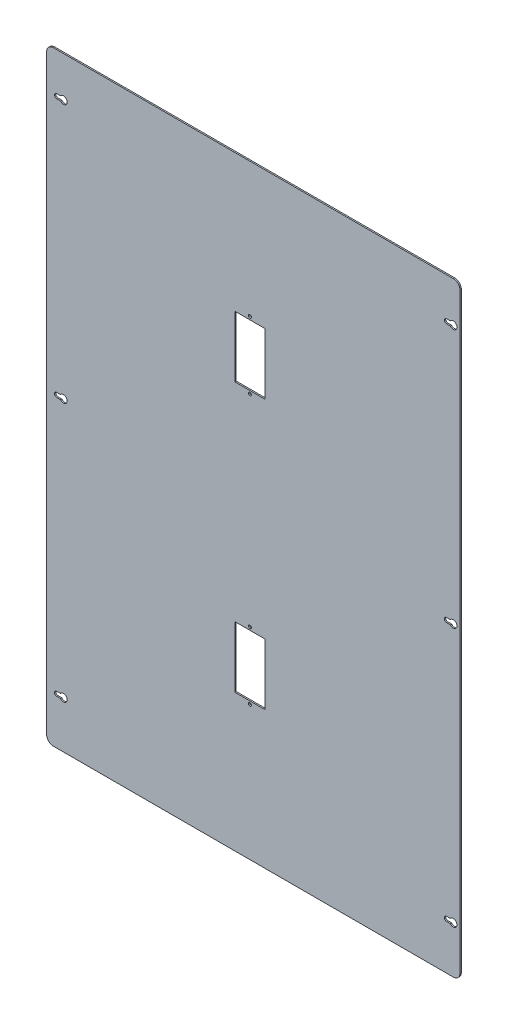
from build123d import *

# Parameters (mm, degrees)
SKETCH1_W            = 615
SKETCH1_H            = 900
BOSS_EXTRUDE1_DEPTH  = 2
SKETCH7_W            = 45
SKETCH7_H            = 91
CUT_EXTRUDE4_DEPTH   = 546.03233849
SKETCH8_R            = 2.25
CUT_EXTRUDE5_DEPTH   = 546.03233849
FILLET3_R            = 10
CUT_EXTRUDE6_DEPTH   = 10
LPATTERN1_COUNT      = 3
LPATTERN1_PITCH      = 385
LPATTERN1_COUNT_DIR2 = 2
LPATTERN1_PITCH_DIR2 = 580


with BuildPart() as part:
    # Sketch1 → Boss-Extrude1 (new body)
    with BuildSketch(Plane.XY):
        Rectangle(SKETCH1_W, SKETCH1_H)
    extrude(amount=BOSS_EXTRUDE1_DEPTH)

    # Sketch7 → Cut-Extrude4 (cut, through all)
    with BuildSketch(Plane(origin=(0, 0, 0), x_dir=(-1, 0, 0), z_dir=(0, 0, -1))):
        with Locations((5, 200)):
            Rectangle(SKETCH7_W, SKETCH7_H)
        with Locations((5, -200)):
            Rectangle(SKETCH7_W, SKETCH7_H)
    extrude(amount=-CUT_EXTRUDE4_DEPTH, mode=Mode.SUBTRACT)

    # Sketch8 → Cut-Extrude5 (cut, through all)
    with BuildSketch(Plane(origin=(0, 0, 0), x_dir=(-1, 0, 0), z_dir=(0, 0, -1))):
        with Locations((5, 250)):
            Circle(SKETCH8_R)
        with Locations((5, 150)):
            Circle(SKETCH8_R)
        with Locations((5, -150)):
            Circle(SKETCH8_R)
        with Locations((5, -250)):
            Circle(SKETCH8_R)
    extrude(amount=-CUT_EXTRUDE5_DEPTH, mode=Mode.SUBTRACT)

    # Fillet3
    fillet3_edges = [part.edges().sort_by_distance(p)[0] for p in [
        (307.5, -450, 1),
        (-307.5, -450, 1),
        (-307.5, 450, 1),
        (307.5, 450, 1),
    ]]
    fillet(fillet3_edges, radius=FILLET3_R)

    # Sketch10 → Cut-Extrude6 (cut)
    with BuildSketch(Plane(origin=(0, 0, 0), x_dir=(-1, 0, 0), z_dir=(0, 0, -1))):
        with BuildLine():
            Line((292.5, 393.3), (286.9, 393.3))
            ThreePointArc((286.9, 393.3), (277, 390), (286.9, 386.7))
            Line((286.9, 386.7), (292.5, 386.7))
            ThreePointArc((292.5, 386.7), (295.8, 390), (292.5, 393.3))
        make_face()
    cut_extrude6 = extrude(amount=-CUT_EXTRUDE6_DEPTH, mode=Mode.SUBTRACT)

    # LPattern1: Cut-Extrude6 3 × 2
    with Locations(*[(j * LPATTERN1_PITCH_DIR2, -i * LPATTERN1_PITCH, 0) for i in range(LPATTERN1_COUNT) for j in range(LPATTERN1_COUNT_DIR2) if (i, j) != (0, 0)]):
        add(cut_extrude6, mode=Mode.SUBTRACT)


solid = part.part
